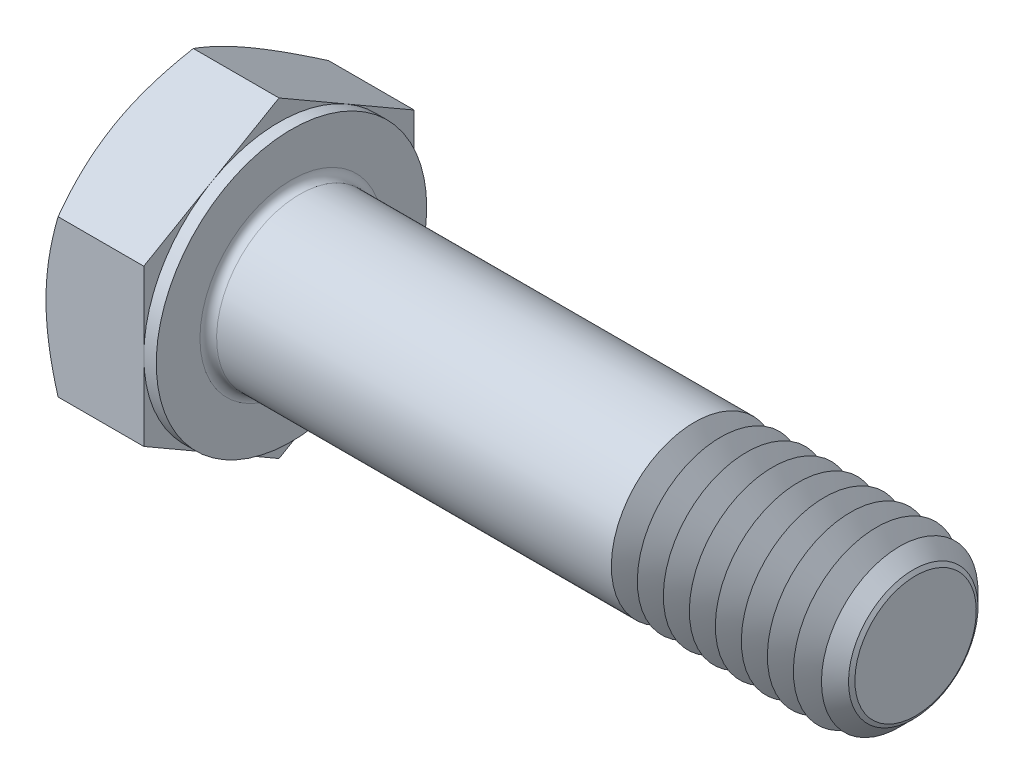
SolidWorks part; units mm, degrees
extrude "基体-拉伸" add sketch "草图1" along normal blind 5.3
sketch "草图1" plane through (0, 0, 0) normal (1, 0, 0) x (0, 0, -1)
  line L0 (6.5, 3.7528) -> (6.5, -3.7528)
  line L1 (-6.5, 3.7528) -> (-6.5, -3.7528)
  line L2 (6.5, -3.7528) -> (0, -7.5056)
  line L3 (0, -7.5056) -> (-6.5, -3.7528)
  line L4 (6.5, 3.7528) -> (0, 7.5056)
  line L5 (0, 7.5056) -> (-6.5, 3.7528)
revolve "切除-旋转1" cut sketch "草图3" angle 360 about L6
sketch "草图3" plane through (0, 0, 0) normal (0, 0, 1) x (1, 0, 0)
  line L0 (0, 6.5) -> (3.4673, 12.5056)
  line L1 (0, 7.5056) -> (0, 3.7528) construction
  line L2 (3.4673, 12.5056) -> (3.4673, 17.5056)
  line L3 (3.4673, 17.5056) -> (-10, 17.5056)
  line L4 (-10, 17.5056) -> (-10, 6.5)
  line L5 (-10, 6.5) -> (0, 6.5)
  line L6 (0, 0) -> (99.06, 0) construction
  line L7 (5.3, 7.5056) -> (0, 7.5056) construction
material "5.6级"
ref_plane "前视" through (0, 0, 0) normal (0, 0, 1) x (1, 0, 0)
ref_plane "上视" through (0, 0, 0) normal (0, 1, 0) x (1, 0, 0)
ref_plane "右视" through (0, 0, 0) normal (1, 0, 0) x (0, 0, -1)
sketch "草图2" plane through (0, 0, 0) normal (0, 0, 1) x (1, 0, 0)
  line L0 (0, 3.7528) -> (0, -3.7528) construction
  line L1 (0, 0) -> (35.3, 0)
  line L2 (0, 0) -> (0, 4)
  line L3 (0, 4) -> (7.7917, 4)
  line L4 (35.3, 0) -> (35.3, 2.9175)
  line L5 (5.3, 7.5056) -> (5.3, 3.7528) construction
  line L7 (0, 0) -> (96.52, 0) construction
  line L8 (35.3, -2.9175) -> (7.7917, -4) construction
  line L9 (0, -4) -> (7.7917, -4) construction
  line L10 (6.55, 15.24) -> (6.55, -1.27) construction
  line L11 (25.3, 15.24) -> (25.3, -1.27) construction
  line L12 (5.3, 3.7528) -> (5.3, -3.7528) construction
  line L13 (7.7917, 4) -> (35.3, 4)
  line L14 (35.3, 4) -> (35.3, 2.9175)
revolve "凸台-旋转1" add sketch "草图2" angle 360 about L7
cosmetic thread "螺旋线1" parameters "Thread_length"=10, "Thread_minor"=5.835
sketch "草图5" plane through (0, 0, 0) normal (0, 0, 1) x (1, 0, 0)
  line L0 (5.3, 6.5) -> (1.8327, 12.5056)
  line L1 (5.3, 7.5056) -> (5.3, 3.7528) construction
  line L2 (1.8327, 12.5056) -> (1.8327, 17.5056)
  line L3 (1.8327, 17.5056) -> (11.8327, 17.5056)
  line L4 (11.8327, 17.5056) -> (11.8327, 6.5)
  line L5 (11.8327, 6.5) -> (5.3, 6.5)
  line L7 (5.3, 7.5056) -> (0.5806, 7.5056) construction
  line L8 (0, 0) -> (99.06, 0) construction
  line L9 (0, 0) -> (99.06, 0) construction
revolve "切除-旋转2" cut sketch "草图5" angle 360 about L8
sketch "草图4" plane through (0, 0, 0) normal (0, 0, 1) x (1, 0, 0)
  line L1 (5.3, 7.5056) -> (5.3, 3.7528) construction
  line L2 (5.3, 6.5) -> (4.7, 6.5)
  line L3 (5.3, 6.5) -> (5.3, 17.5056)
  line L4 (5.3, 17.5056) -> (4.7, 17.5056)
  line L5 (0, 0) -> (95.25, 0) construction
  line L6 (0, 0) -> (96.52, 0) construction
  line L7 (4.7, 6.5) -> (4.7, 17.5056)
  line L8 (4.7194, 7.5056) -> (0.5806, 7.5056) construction
revolve "切除-旋转3" cut sketch "草图4" angle 360 about L5
chamfer "倒角" distance 1 angle 45 1 edges at (35.3, 0, 4)
fillet "圆角" radius 0.4 1 edges at (5.3, 0, -4)
sketch "草图6" plane through (0, 0, 0) normal (0, 0, 1) x (1, 0, 0)
  line L0 (25.3, -2.9175) -> (24.675, -4)
  line L1 (25.3, -2.9175) -> (25.925, -4)
  line L2 (25.925, -4) -> (25.925, -5)
  line L3 (-3.175, 0) -> (5.1513, 0) construction
  line L5 (25.925, -5) -> (24.675, -5)
  line L6 (24.675, -5) -> (24.675, -4)
revolve "切除-旋转4" cut sketch "草图6" angle 360 about L3
pattern_linear "阵列(线性)1" count 9 spacing 1.25 along (1, 0, 0) of "切除-旋转4"
equation "\"D3@草图1\" = \"s@草图1\" / 2"
equation "\"D4@草图1\" = \"D3@草图1\""
equation "\"D5@草图1\" = \"D4@草图1\""
equation "\"Thread_minor@螺旋线1\" = \"Minor_dia@草图2\""
equation "\"D1@草图3\" = \"s@草图1\" / 2"
equation "\"D1@草图5\" = \"s@草图1\" / 2"
equation "\"Head_ch_ang@草图5\" = \"Head_ch_ang@草图3\""
equation "\"D1@草图4\" = \"s@草图1\""
equation "\"Thread_length@螺旋线1\" = ((sgn( (\"l@草图2\" - \"p@草图2\" ) - \"h@草图2\" )-1)*( (\"l@草图2\" - \"p@草图2\" ) - \"h@草图2\" ))/-2+ \"h@草图2\""
equation "\"Thread_minor@草图6\" = \"Minor_dia@草图2\""
equation "\"Diameter@草图6\" = \"m@草图2\""
equation "\"Overcut@草图6\" = \"m@草图2\" * 1.25"
equation "\"Start@草图6\" = \"k@基体-拉伸\" + \"l@草图2\" - \"Thread_length@螺旋线1\"  '---Non-countersunk---"
equation "\"Num_threads@阵列(线性)1\" = int( \"Thread_length@螺旋线1\" / \"p@草图2\" + 0.999 )  + 1"
equation "\"Advance@阵列(线性)1\" = \"Thread_length@螺旋线1\" /  (\"Num_threads@阵列(线性)1\" - 1) 'relax it"
equation "\"Num_threads@阵列(线性)1\" = \"Num_threads@阵列(线性)1\" - sgn( \"Num_threads@阵列(线性)1\" - 1) '---chamfered tips only---"
equation "\"Minor_dia@草图2\" = \"m@草图2\"-\"p@草图2\" * 1.732"
equation "\"D1@倒角\" = \"p@草图2\"*0.8"
